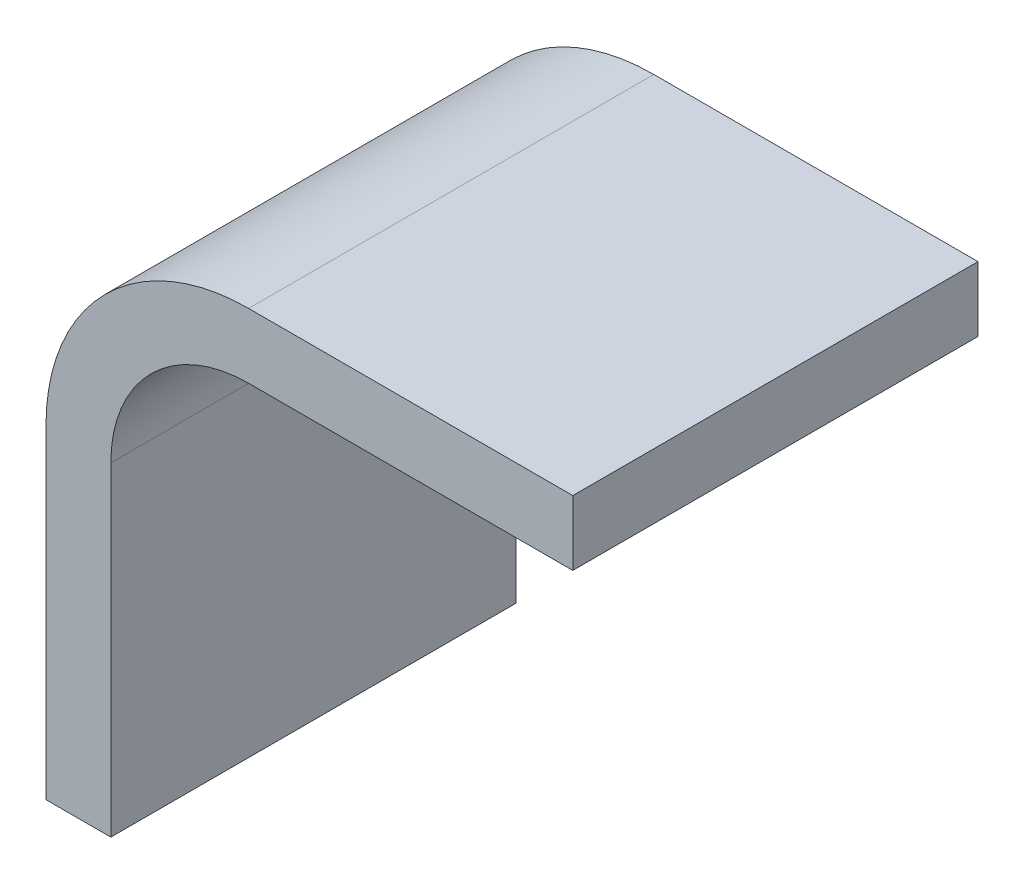
from build123d import *

# Parameters (mm, degrees)
EXTRUDE_THIN1_DEPTH = 100


with BuildPart() as part:
    # Sketch1 → Extrude-Thin1 (new body)
    with BuildSketch(Plane.XY):
        with BuildLine():
            Line((0, -130), (0, -50))
            ThreePointArc((0, -50), (14.644660941, -14.644660941), (50, 0))
            Line((50, 0), (130, 0))
            Line((130, 0), (130, -16))
            Line((130, -16), (50, -16))
            ThreePointArc((50, -16), (25.95836944, -25.95836944), (16, -50))
            Line((16, -50), (16, -130))
            Line((16, -130), (0, -130))
        make_face()
    extrude(amount=EXTRUDE_THIN1_DEPTH)


solid = part.part
